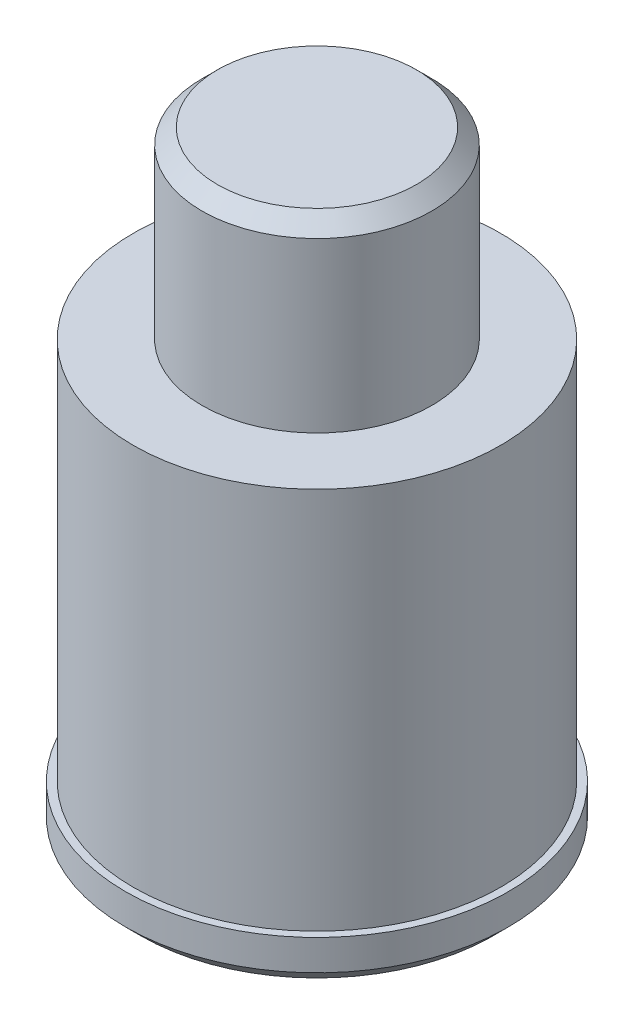
from build123d import *

# Parameters (mm, degrees)
SKETCH1_R           = 12.5
BOSS_EXTRUDE1_DEPTH = 3
SKETCH2_R           = 12
BOSS_EXTRUDE2_DEPTH = 25
SKETCH3_R           = 7.5
BOSS_EXTRUDE3_DEPTH = 12
CUT_EXTRUDE1_DEPTH  = 4
CHAMFER1_SIZE       = 1


with BuildPart() as part:
    # Sketch1 → Boss-Extrude1 (new body)
    with BuildSketch(Plane(origin=(0, 0, 0), x_dir=(1, 0, 0), z_dir=(0, 1, 0))):
        with Locations(Location((0, 0, 0), (0, 0, 270))):
            Circle(SKETCH1_R)
    extrude(amount=BOSS_EXTRUDE1_DEPTH)

    # Sketch2 → Boss-Extrude2 (add)
    with BuildSketch(Plane(origin=(0, 3, 0), x_dir=(1, 0, 0), z_dir=(0, 1, 0))):
        with Locations(Location((0, 0, 0), (0, 0, 270))):
            Circle(SKETCH2_R)
    extrude(amount=BOSS_EXTRUDE2_DEPTH)

    # Sketch3 → Boss-Extrude3 (add)
    with BuildSketch(Plane(origin=(0, 28, 0), x_dir=(1, 0, 0), z_dir=(0, 1, 0))):
        with Locations(Location((0, 0, 0), (0, 0, 270))):
            Circle(SKETCH3_R)
    extrude(amount=BOSS_EXTRUDE3_DEPTH)

    # Sketch4 → Cut-Extrude1 (cut)
    with BuildSketch(Plane(origin=(0, 0, -12), x_dir=(-1, 0, 0), z_dir=(0, 0, -1))):
        with BuildLine():
            Line((4, 23), (4, 8))
            ThreePointArc((4, 8), (0, 4), (-4, 8))
            Line((-4, 8), (-4, 23))
            ThreePointArc((-4, 23), (0, 27), (4, 23))
        make_face()
    extrude(amount=-CUT_EXTRUDE1_DEPTH, mode=Mode.SUBTRACT)

    # Chamfer1
    chamfer1_edges = [part.edges().sort_by_distance(p)[0] for p in [
        (0, 40, -7.5),
        (0, 0, -12.5),
    ]]
    chamfer(chamfer1_edges, length=CHAMFER1_SIZE)


solid = part.part
